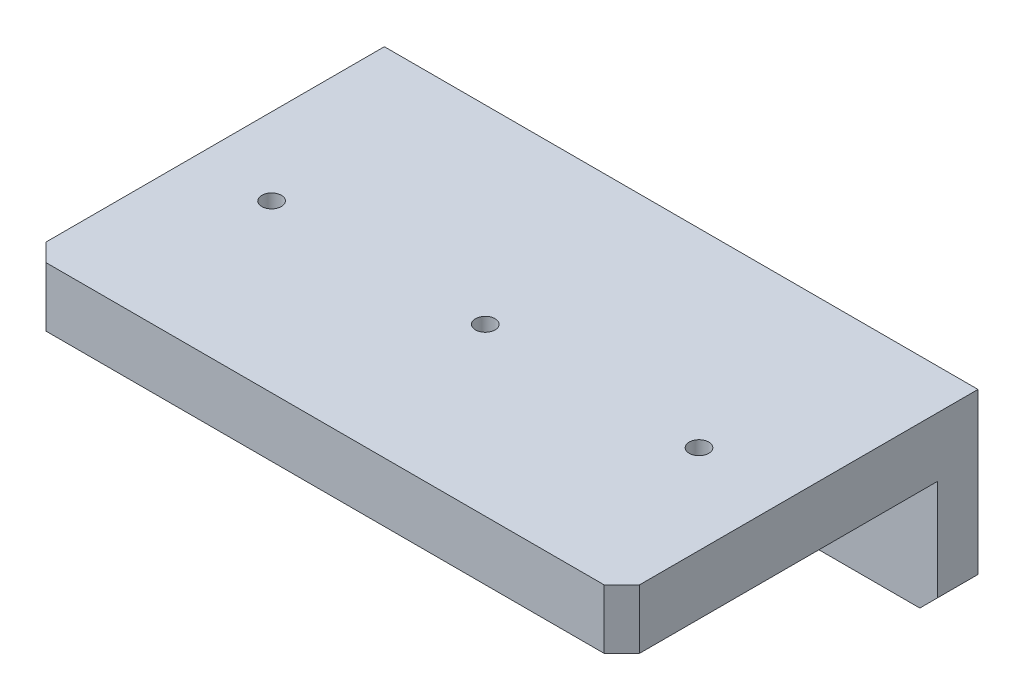
SolidWorks part; units mm, degrees
material "A6061 T6"
ref_plane "前视基准面" through (0, 0, 0) normal (0, 0, 1) x (1, 0, 0)
ref_plane "上视基准面" through (0, 0, 0) normal (0, 1, 0) x (1, 0, 0)
ref_plane "右视基准面" through (0, 0, 0) normal (1, 0, 0) x (0, 0, -1)
sketch "草图1" plane through (0, 0, 0) normal (0, 1, 0) x (1, 0, 0)
  line L1 (-50, 30) -> (50, 30)
  line L2 (-50, 30) -> (-50, -30)
  line L3 (-50, -30) -> (50, -30)
  line L4 (50, 30) -> (50, -30)
  line L5 (-50, 30) -> (50, -30) construction
  line L6 (-50, -30) -> (50, 30) construction
  point P0 (0, 0)
  dimension "D1" = 100
  dimension "D2" = 60
extrude "凸台-拉伸1" add sketch "草图1" along normal blind 10
sketch "草图2" plane through (0, 0, 0) normal (0, -1, 0) x (1, 0, 0)
  line L0 (-50, -30) -> (-50, 30) construction
  line L1 (50, -30) -> (-50, -30)
  line L2 (50, -30) -> (50, -23.2)
  line L3 (50, -23.2) -> (-50, -23.2)
  line L4 (-50, -30) -> (-50, -23.2)
  dimension "D1" = 6.8
extrude "凸台-拉伸2" add sketch "草图2" along normal blind 20
chamfer "倒角1" distance 3 angle 45 4 edges at (-50, -20, -26.6) (-50, 5, 30) (50, 5, 30) (50, -20, -26.6)
hole_wizard "M4 螺纹孔1" positions "草图3" profile "草图4" tap size "M4" standard "GB"
sketch "草图3" plane through (0, 10, 0) normal (0, 1, 0) x (1, 0, 0)
  point P0 (35, -2)
  point P3 (-37, -2)
  point P6 (-1, -2)
sketch "草图4" plane through (35, 10, 2) normal (1, 0, 0) x (0, 0, 1)
  line L0 (0, 0) -> (0, 11.0914)
  line L1 (0, 11.0914) -> (1.65, 10.1)
  line L2 (1.65, 10.1) -> (1.65, 0)
  line L5 (1.65, 0) -> (0, 0)
  line L10 (0, 11.0914) -> (-1.65, 10.1) construction
  line L11 (0, -6.35) -> (0, 107.95) construction
  dimension "螺纹孔钻头直径" = 3.3
  dimension "螺纹孔钻头深度" = 10.1
  dimension "导头角度" = 118
cosmetic thread "孔螺蚊线1"
cosmetic thread "孔螺蚊线2"
cosmetic thread "孔螺蚊线3"
hole_wizard "打孔尺寸(%根据)开槽半沉头木螺钉的类型1" positions "草图5" profile "草图6" countersink size "M5" standard "GB"
sketch "草图5" plane through (0, 0, -23.2) normal (0, 0, 1) x (1, 0, 0)
  line L0 (47, -20) -> (-47, -20) construction
  line L1 (50, -17) -> (50, 0) construction
  point P0 (-10, -10)
  point P2 (-25, -10)
  dimension "D1" = 10
  dimension "D2" = 15
  dimension "D3" = 60
sketch "草图6" plane through (-10, -10, -23.2) normal (1, 0, 0) x (0, -1, 0)
  line L0 (0, 0) -> (0, 11.7524)
  line L1 (0, 11.7524) -> (2.75, 10.1)
  line L2 (2.75, 10.1) -> (2.75, 2.85)
  line L3 (2.75, 2.85) -> (5.6, 0)
  line L5 (5.6, 0) -> (0, 0)
  line L6 (-2.75, 2.85) -> (-5.6, 0) construction
  line L10 (0, 11.7524) -> (-2.75, 10.1) construction
  line L11 (0, -6.35) -> (0, 107.95) construction
  dimension "孔直径" = 5.5
  dimension "孔深度" = 10.1
  dimension "近端锥形沉头孔直径" = 11.2
  dimension "近端锥形沉头孔角度" = 90
  dimension "导头角度" = 118
